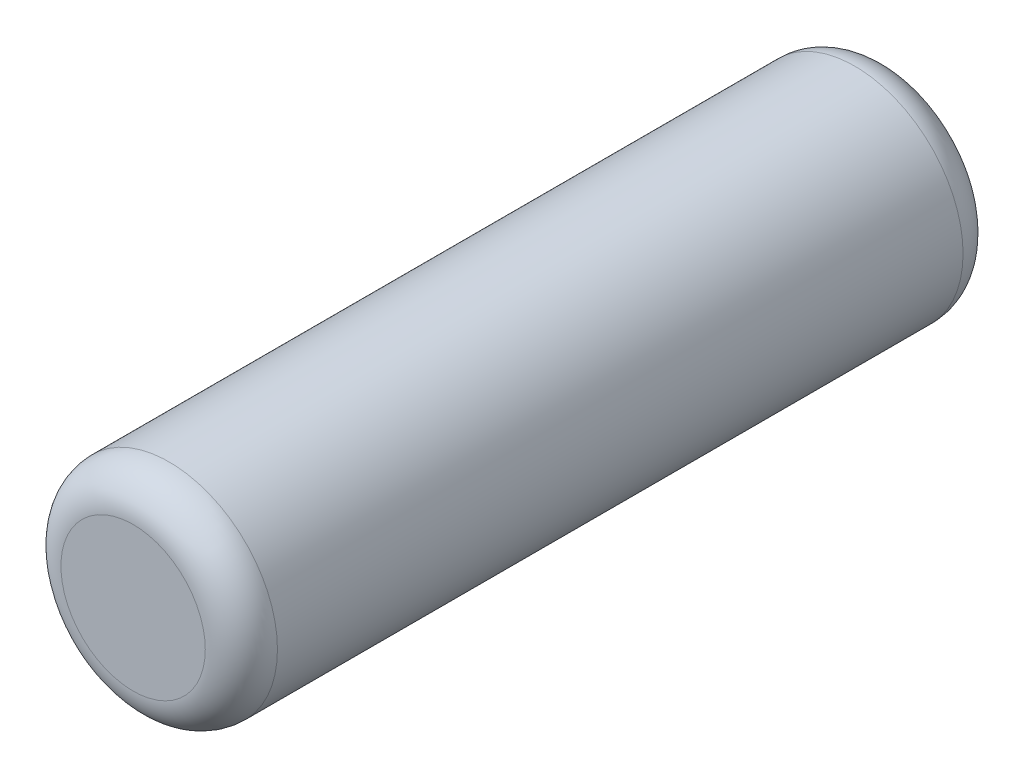
SolidWorks part; units mm, degrees
ref_plane "Front Plane" through (0, 0, 0) normal (0, 0, 1) x (1, 0, 0)
ref_plane "Top Plane" through (0, 0, 0) normal (0, 1, 0) x (1, 0, 0)
ref_plane "Right Plane" through (0, 0, 0) normal (1, 0, 0) x (0, 0, -1)
other "Configuration Table"
sketch "Sketch1" plane through (0, 0, 0) normal (0, 0, 1) x (1, 0, 0)
  circle A0 centre (0, 0) radius 3
  dimension "D1" = 6
extrude "Boss-Extrude1" add sketch "Sketch1" along normal blind 21
fillet "Fillet1" radius 1 2 edges at (3, 0, 0) (3, 0, 21)
